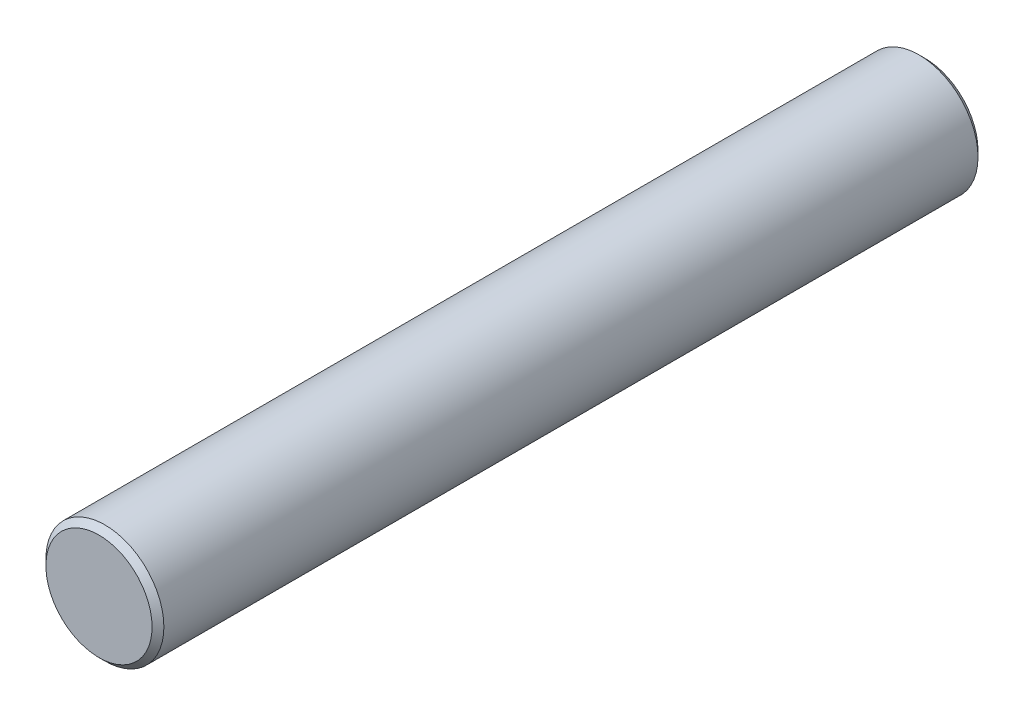
SolidWorks part; units mm, degrees
ref_plane "Front Plane" through (0, 0, 0) normal (0, 0, 1) x (1, 0, 0)
ref_plane "Top Plane" through (0, 0, 0) normal (0, 1, 0) x (1, 0, 0)
ref_plane "Right Plane" through (0, 0, 0) normal (1, 0, 0) x (0, 0, -1)
sketch "Sketch1" plane through (0, 0, 0) normal (0, 0, 1) x (1, 0, 0)
  circle A0 centre (0, 0) radius 10
  dimension "D1" = 20
extrude "Boss-Extrude1" add sketch "Sketch1" against normal blind 140
cosmetic thread "Cosmetic Thread1" parameters "D1"=40, "D2"=17.294
cosmetic thread "Cosmetic Thread2" parameters "D1"=40, "D2"=17.294
chamfer "Chamfer2" distance 1 angle 45 2 edges at (10, 0, -140) (10, 0, 0)
